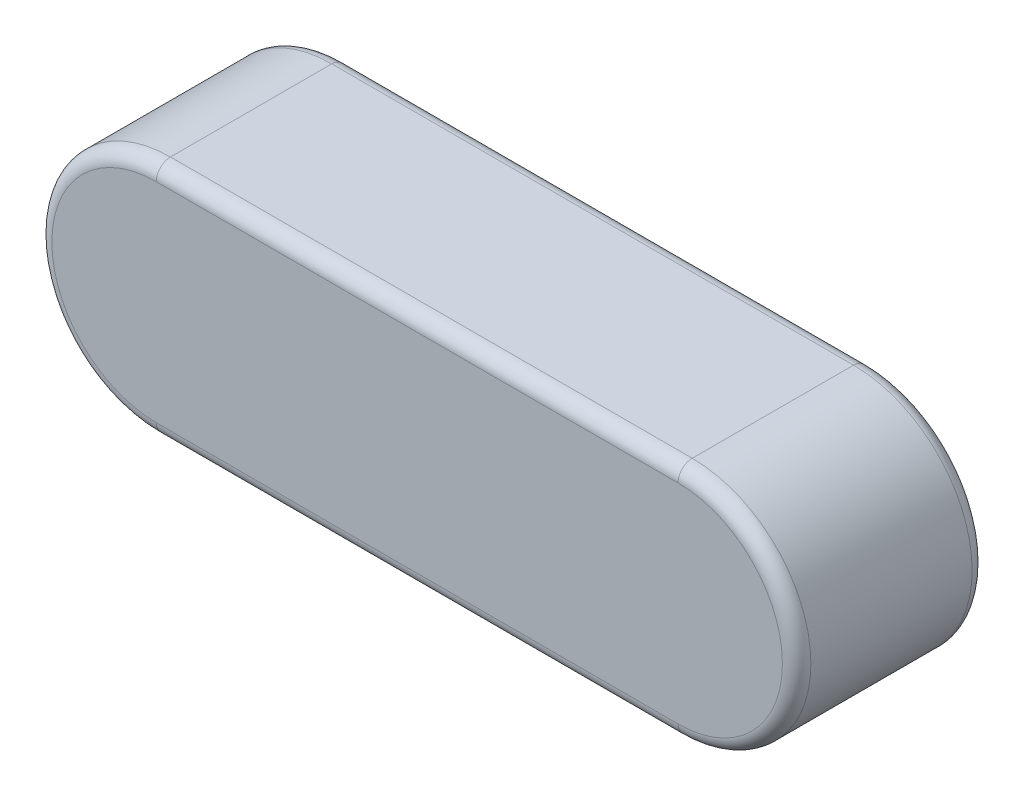
SolidWorks part; units mm, degrees
material "45"
ref_plane "基准面1" through (0, 0, 0) normal (0, 0, 1) x (1, 0, 0)
ref_plane "基准面2" through (0, 0, 0) normal (0, 1, 0) x (1, 0, 0)
ref_plane "基准面3" through (0, 0, 0) normal (1, 0, 0) x (0, 0, -1)
sketch "尺寸草图" plane through (0, 0, 0) normal (0, 0, 1) x (1, 0, 0)
  line L0 (-16, 0) -> (16, 0) construction
  point P3 (-8, 0)
  point P4 (-0.6, 0)
  point P5 (0, 0)
  point P8 (-10, 0)
  point P11 (0, 0)
sketch "草图1" plane through (0, 0, 0) normal (0, 0, 1) x (1, 0, 0)
  line L0 (-28.0599, 0) -> (30.562, 0) construction
  line L1 (-11, 5) -> (11, 5)
  line L2 (-11, -5) -> (11, -5)
  line L3 (0, 2.9108) -> (0, -2.1805) construction
  arc A0 (-11, 5) -> (-11, -5) centre (-11, 0) ccw
  arc A1 (11, 5) -> (11, -5) centre (11, 0) cw
extrude "基体-拉伸" add sketch "草图1" along normal blind 8
fillet "圆角1" radius 0.6 8 edges at (16, 0, 8) (0, 5, 8) (-16, 0, 8) (0, 5, 0) (16, 0, 0) (0, -5, 0) (-16, 0, 0) (0, -5, 8)
equation "\"D3@草图1\" = \"L@尺寸草图\""
equation "\"D1@草图1\" = \"b@尺寸草图\" / 2"
equation "\"D1@圆角1\" = \"r@尺寸草图\""
equation "\"D1@基体-拉伸\" = \"h@尺寸草图\""
